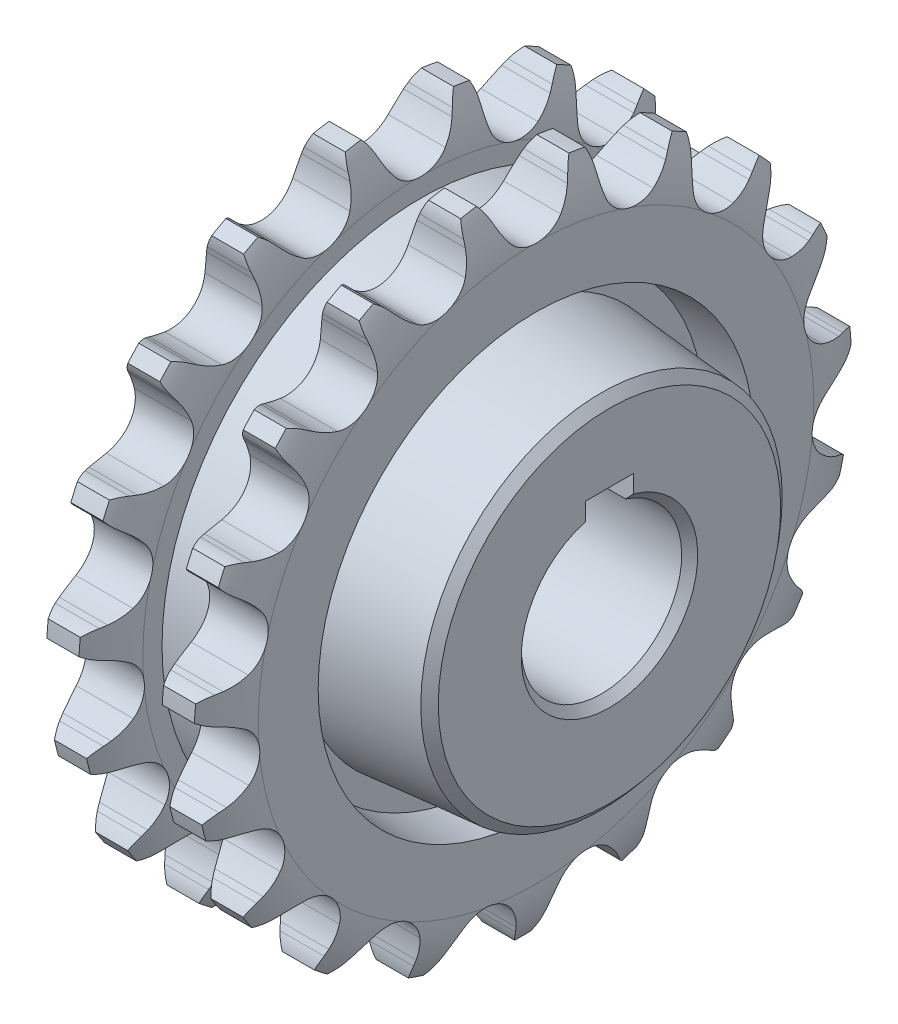
from build123d import *
from OCP.BRepFilletAPI import BRepFilletAPI_MakeChamfer

# Parameters (mm, degrees)
CUT_EXTRUDE1_DEPTH = 5.475375
CIRPATTERN1_COUNT  = 19
LPATTERN1_COUNT    = 2
LPATTERN1_PITCH    = 14.38
CHAMFER1_SIZE      = 1
CHAMFER1_SIZE2     = 1.100062868
SKETCH4_W          = 6
SKETCH4_H          = 3.260607986
CUT_EXTRUDE4_DEPTH = 71.401283385


with BuildPart() as part:
    # Sketch1 → Revolve1 (revolve)
    with BuildSketch(Plane.XY, mode=Mode.PRIVATE) as revolve1_sk:
        with BuildLine():
            Line((-3.65025, 27.149639763), (-3.65025, 34.619639763))
            ThreePointArc((-3.65025, 34.619639763), (-3.245836945, 37.918781526), (-1.99925, 41))
            Line((-1.99925, 41), (1.99925, 41))
            ThreePointArc((1.99925, 41), (3.245836945, 37.918781526), (3.65025, 34.619639763))
            Line((3.65025, 34.619639763), (3.65025, 27.149639763))
            Line((3.65025, 27.149639763), (-3.65025, 27.149639763))
        make_face()
    revolve(revolve1_sk.sketch.rotate(Axis((-6.35, 0, 0), (1, 0, 0)), 90), axis=Axis((-6.35, 0, 0), (1, 0, 0)))

    # Sketch2 → Cut-Extrude1 (cut, symmetric)
    with BuildSketch(Plane(origin=(0, 0, 0), x_dir=(0, 0, -1), z_dir=(1, 0, 0))):
        with BuildLine():
            Line((4.552244709, 38.426451297), (4.858741585, 39.1448403))
            ThreePointArc((4.858741585, 39.1448403), (5.250930322, 39.90290393), (5.750855114, 40.594675334))
            ThreePointArc((5.750855114, 40.594675334), (0, 41), (-5.750855114, 40.594675334))
            ThreePointArc((-5.750855114, 40.594675334), (-5.250930322, 39.90290393), (-4.858741585, 39.1448403))
            Line((-4.858741585, 39.1448403), (-4.552244709, 38.426451297))
            ThreePointArc((-4.552244709, 38.426451297), (-3.937302758, 37.212676935), (-3.168676608, 36.089905522))
            ThreePointArc((-3.168676608, 36.089905522), (0, 34.549839763), (3.168676608, 36.089905522))
            ThreePointArc((3.168676608, 36.089905522), (3.937302758, 37.212676935), (4.552244709, 38.426451297))
        make_face()
    cut_extrude1 = extrude(amount=CUT_EXTRUDE1_DEPTH, both=True, mode=Mode.SUBTRACT)

    # CirPattern1: Cut-Extrude1 ×19 about axis
    cirpattern1_axis = Axis((0, 0, 0), (1, 0, 0))
    for i in range(1, CIRPATTERN1_COUNT):
        add(cut_extrude1.rotate(cirpattern1_axis, i * 360 / CIRPATTERN1_COUNT), mode=Mode.SUBTRACT)


with BuildPart() as lpattern1_1:
    # LPattern1: pattern copy
    add(part.part.moved(Location(Vector(1, 0, 0) * (1 * LPATTERN1_PITCH))))


with BuildPart() as part_1:
    add(part.part)

    # Sketch5 → Revolve2 (revolve)
    with BuildSketch(Plane.XY, mode=Mode.PRIVATE) as revolve2_sk:
        Polygon((-12.81, 10), (27.19, 10), (27.19, 22.438259462), (12.34, 23.737466115), (12.34, 26.651807396), (18.03025, 27.149639763), (10.72975, 32.229639763), (3.65025, 32.229639763), (-3.65025, 27.149639763), (2.04, 26.651807396), (2.04, 23.737466115), (-12.81, 22.438259462), align=None)
    revolve(revolve2_sk.sketch.rotate(Axis((0, 0, 0), (-1, 0, 0)), 90), axis=Axis((0, 0, 0), (-1, 0, 0)))

    # Chamfer1: one chamfer whose edges measure the first distance from different faces: ONE call of the kernel's chamfer builder (chamfer() names one face for all edges)
    chamfer1_edges_1 = [part_1.edges().sort_by_distance(p)[0] for p in [
        (-12.81, 0, 10),
        (27.19, 0, 10),
    ]]
    chamfer1_edges_2 = [part_1.edges().sort_by_distance(p)[0] for p in [
        (-12.81, 0, 22.438259462),
    ]]
    chamfer1_side_2 = [part_1.faces().sort_by_distance(p)[0] for p in [
        (-12.81, 0, 21.803609645),
    ]]
    chamfer1_edges_3 = [part_1.edges().sort_by_distance(p)[0] for p in [
        (27.19, 0, 22.438259462),
    ]]
    chamfer1_side_3 = [part_1.faces().sort_by_distance(p)[0] for p in [
        (19.765, 0, 23.087862789),
    ]]
    chamfer1 = BRepFilletAPI_MakeChamfer(part_1.part.solid().wrapped)
    for e in chamfer1_edges_1:
        chamfer1.Add(CHAMFER1_SIZE, e.wrapped)
    for e in chamfer1_edges_2:
        chamfer1.Add(CHAMFER1_SIZE, CHAMFER1_SIZE2, e.wrapped, chamfer1_side_2[0].wrapped)  # the first distance lies on this face
    for e in chamfer1_edges_3:
        chamfer1.Add(CHAMFER1_SIZE, CHAMFER1_SIZE2, e.wrapped, chamfer1_side_3[0].wrapped)  # the first distance lies on this face
    add(Compound.cast(chamfer1.Shape()), mode=Mode.REPLACE)

    # Sketch4 → Cut-Extrude4 (cut, through all)
    with BuildSketch(Plane.ZY.offset(12.81)):
        with Locations((0, 11.169696007)):
            Rectangle(SKETCH4_W, SKETCH4_H)
    extrude(amount=-CUT_EXTRUDE4_DEPTH, mode=Mode.SUBTRACT)


solid = Compound([lpattern1_1.part, part_1.part])
